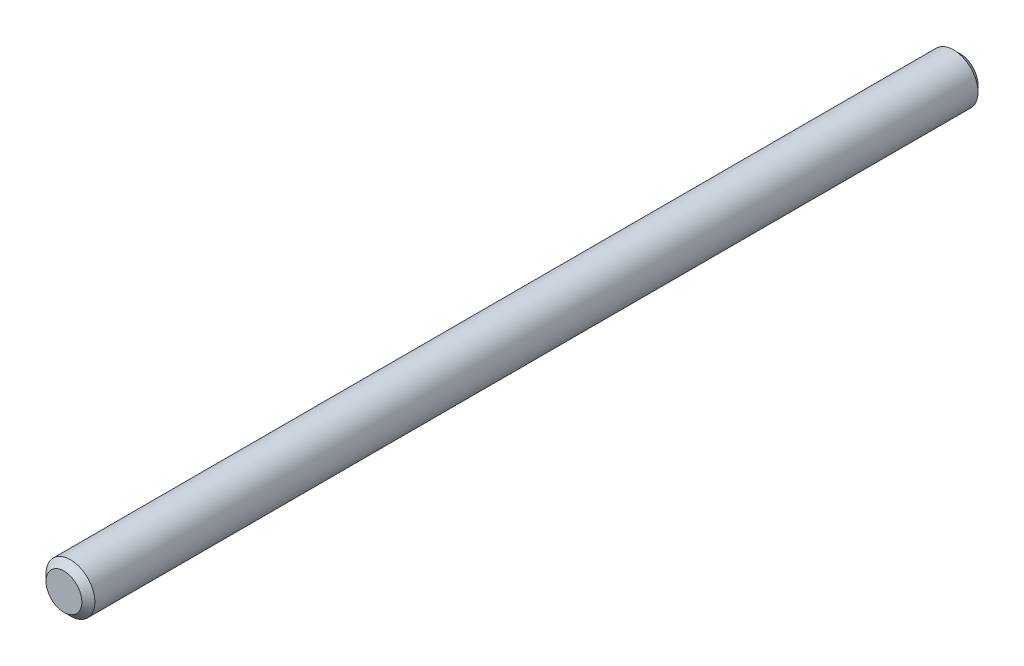
SolidWorks part; units mm, degrees
ref_plane "Front Plane" through (0, 0, 0) normal (0, 0, 1) x (1, 0, 0)
ref_plane "Top Plane" through (0, 0, 0) normal (0, 1, 0) x (1, 0, 0)
ref_plane "Right Plane" through (0, 0, 0) normal (1, 0, 0) x (0, 0, -1)
sketch "Sketch1" plane through (0, 0, 0) normal (0, 0, 1) x (1, 0, 0)
  circle A0 centre (0, 0) radius 0.75
  dimension "D1" = 1.5
extrude "Boss-Extrude1" add sketch "Sketch1" along normal mid plane 27.5
chamfer "Chamfer1" distance 0.2 2 edges at (0.75, 0, -13.75) (0.75, 0, 13.75)
